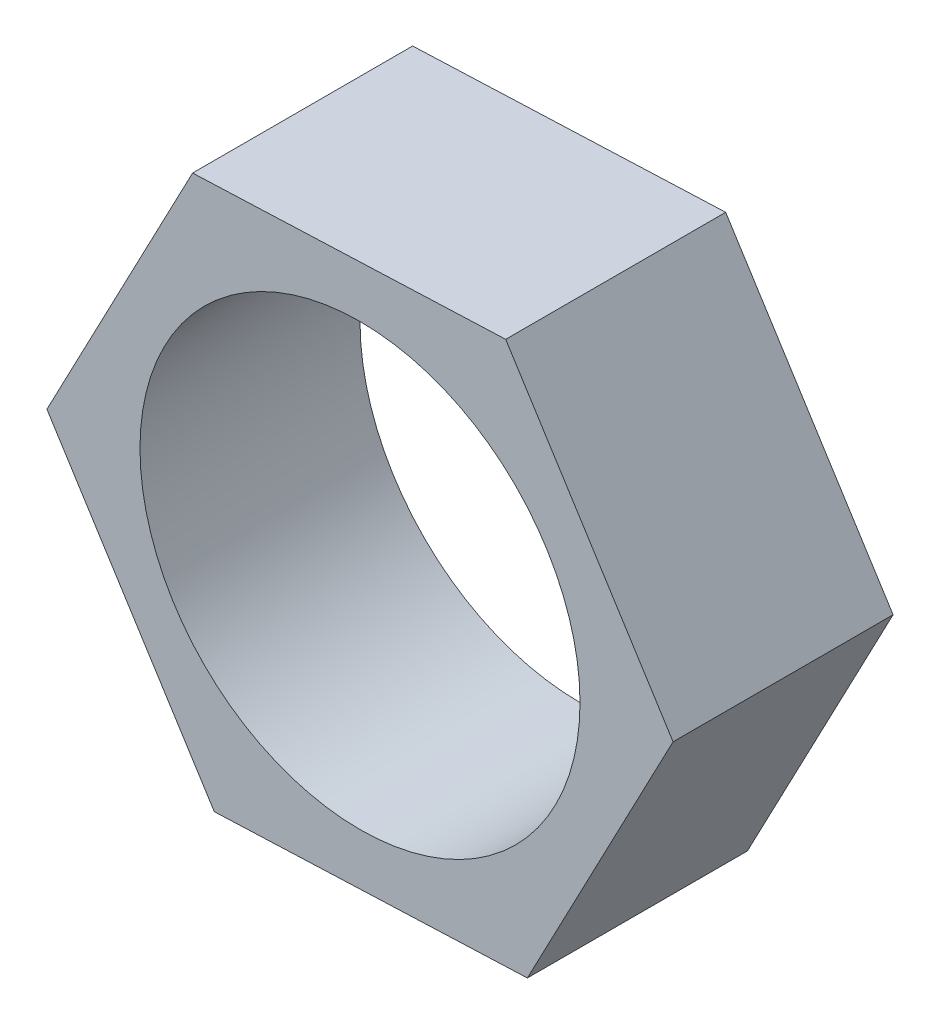
from build123d import *

# Parameters (mm, degrees)
SKETCH1_R           = 15
BOSS_EXTRUDE1_DEPTH = 15


with BuildPart() as part:
    # Sketch1 → Boss-Extrude1 (new body)
    with BuildSketch(Plane.XY):
        Polygon((9.932712467, 18.912285858), (-11.412163764, 18.058124254), (-21.34487623, -0.854161605), (-9.932712467, -18.912285858), (11.412163764, -18.058124254), (21.34487623, 0.854161605), align=None)
        Circle(SKETCH1_R, mode=Mode.SUBTRACT)
    extrude(amount=BOSS_EXTRUDE1_DEPTH)


solid = part.part
